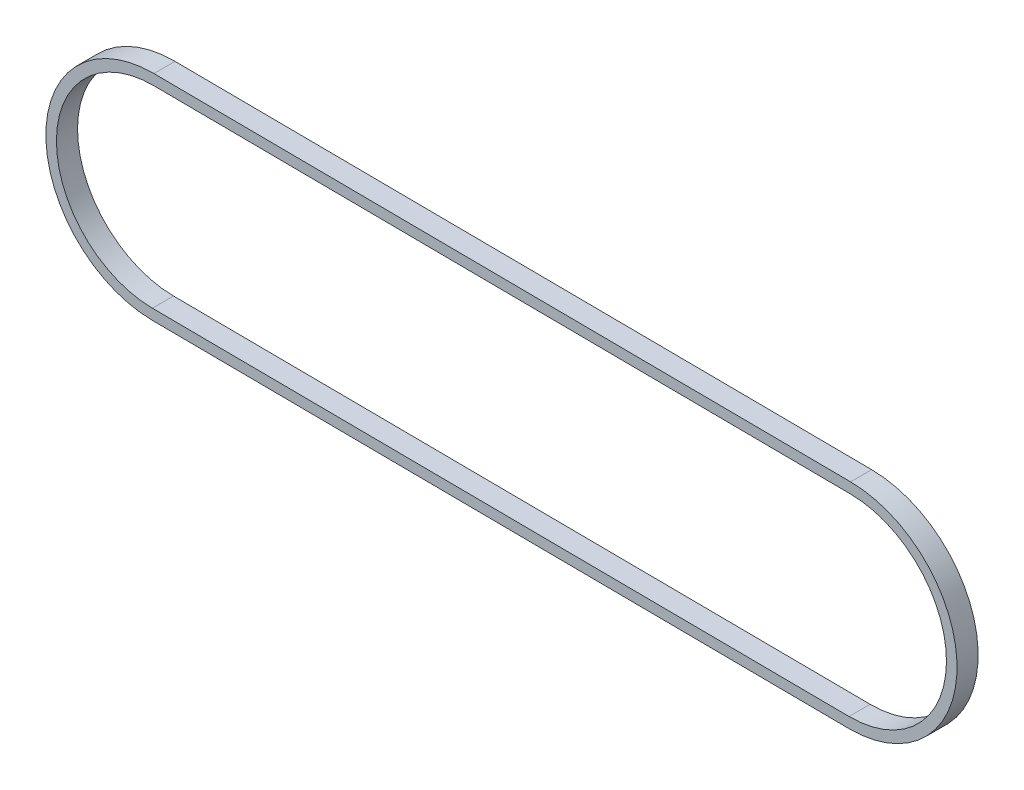
SolidWorks part; units mm, degrees
ref_plane "前视基准面" through (0, 0, 0) normal (0, 0, 1) x (1, 0, 0)
ref_plane "上视基准面" through (0, 0, 0) normal (0, 1, 0) x (1, 0, 0)
ref_plane "右视基准面" through (0, 0, 0) normal (1, 0, 0) x (0, 0, -1)
sketch "草图2" plane through (0, 0, 0) normal (0, 0, 1) x (1, 0, 0)
  line L0 (0, 0) -> (1, 0) construction
  line L1 (0, 0) -> (0, 1) construction
  line L2 (0.6941, 91.6224) -> (660.6941, 86.6224)
  line L3 (659.3059, -96.6224) -> (-0.6941, -91.6224)
  arc A0 (-0.6941, -91.6224) -> (0.6941, 91.6224) centre (0, 0) cw
  arc A1 (660.6941, 86.6224) -> (659.3059, -96.6224) centre (660, -5) cw
extrude "拉伸-薄壁1" add sketch "草图2" along normal mid plane 20 thin thin type one direction wall 10
